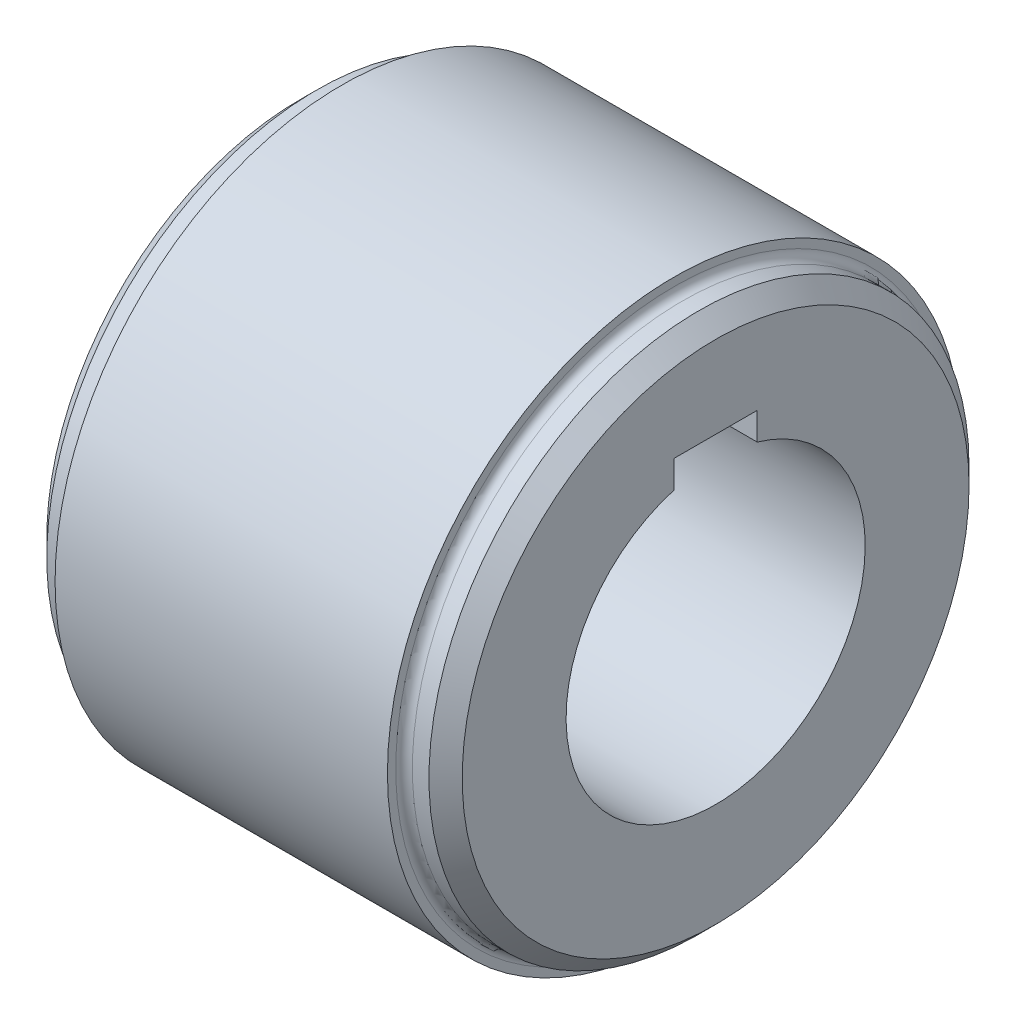
SolidWorks part; units mm, degrees
ref_plane "前视基准面" through (0, 0, 0) normal (0, 0, 1) x (1, 0, 0)
ref_plane "上视基准面" through (0, 0, 0) normal (0, 1, 0) x (1, 0, 0)
ref_plane "右视基准面" through (0, 0, 0) normal (1, 0, 0) x (0, 0, -1)
sketch "草图1" plane through (0, 0, 0) normal (1, 0, 0) x (0, 0, -1)
  line L2 (5, 17.2916) -> (5, 20.5916)
  line L3 (5, 20.5916) -> (-5, 20.5916)
  line L4 (-5, 20.5916) -> (-5, 17.2916)
  arc A0 (-5, 17.2916) -> (5, 17.2916) centre (0, 0) ccw
  circle A1 centre (0, 0) radius 32.5
  dimension "D1" = 3.3
extrude "凸台-拉伸1" add sketch "草图1" along normal mid plane 50
sketch "草图2" plane through (0, 0, 0) normal (1, 0, 0) x (0, 0, -1)
  circle A0 centre (0, 0) radius 32.5
  circle A1 centre (0, 0) radius 34.5
extrude "凸台-拉伸2" add sketch "草图2" along normal mid plane 40
fillet "圆角1" radius 1 2 edges at (-20, 0, -32.5) (20, 0, -32.5)
chamfer "倒角1" distance 2 angle 45 2 edges at (25, 0, -32.5) (-25, 0, -32.5)
